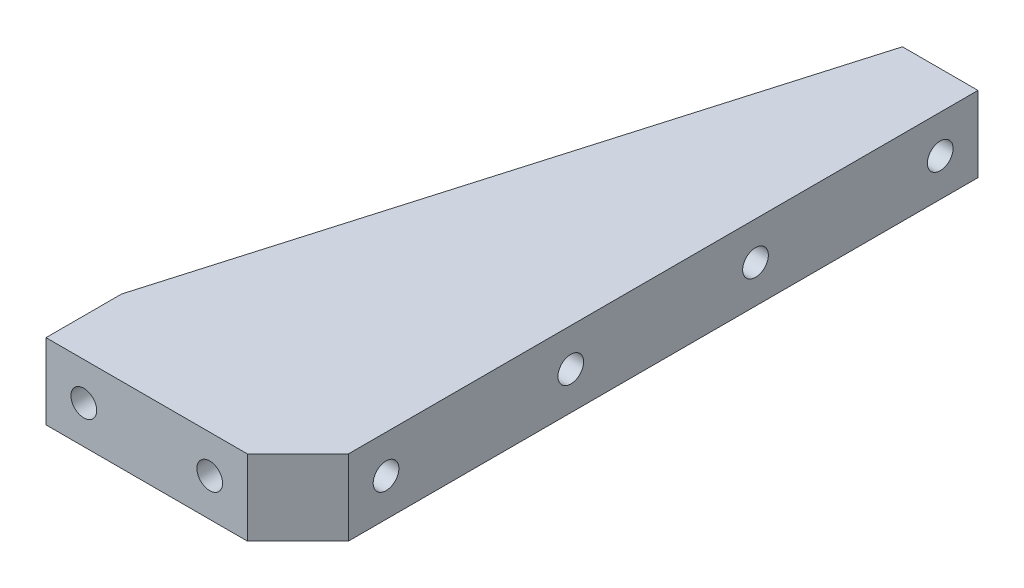
SolidWorks part; units mm, degrees
material "普通碳钢"
ref_plane "前视基准面" through (0, 0, 0) normal (0, 0, 1) x (1, 0, 0)
ref_plane "上视基准面" through (0, 0, 0) normal (0, 1, 0) x (1, 0, 0)
ref_plane "右视基准面" through (0, 0, 0) normal (1, 0, 0) x (0, 0, -1)
sketch "草图1" plane through (0, 0, 0) normal (0, 1, 0) x (1, 0, 0)
  line L0 (0, 0) -> (0, -250)
  line L1 (0, -250) -> (-20, -270)
  line L2 (-20, -270) -> (-100, -270)
  line L3 (-100, -270) -> (-100, -240)
  line L4 (-100, -240) -> (-30, 0)
  line L5 (-30, 0) -> (0, 0)
  dimension "D1" = 270
  dimension "D2" = 100
  dimension "D3" = 30
  dimension "D4" = 30
  dimension "D5" = 45
  dimension "D6" = 20
extrude "凸台-拉伸1" add sketch "草图1" along normal blind 30
hole_wizard "M12 螺纹孔1" positions "草图2" profile "草图3" tap size "M12" standard "GB"
sketch "草图2" plane through (0, 0, 0) normal (1, 0, 0) x (0, 0, -1)
  line L0 (0, 30) -> (0, 0) construction
  line L1 (-250, 30) -> (-250, 0) construction
  line L2 (-15, 15) -> (-88.3333, 15) construction
  line L3 (-88.3333, 15) -> (-161.6667, 15) construction
  line L4 (-161.6667, 15) -> (-235, 15) construction
  point P0 (-235, 15)
  point P2 (-15, 15)
  point P9 (0, 15)
  point P12 (-88.3333, 15)
  point P14 (-161.6667, 15)
  dimension "D1" = 15
  dimension "D2" = 15
sketch "草图3" plane through (0, 15, 235) normal (0, 1, 0) x (0, 0, -1)
  line L0 (0, 0) -> (0, 32.3144)
  line L1 (0, 32.3144) -> (5.1, 29.25)
  line L2 (5.1, 29.25) -> (5.1, 0)
  line L5 (5.1, 0) -> (0, 0)
  line L10 (0, 32.3144) -> (-5.1, 29.25) construction
  line L11 (0, -6.35) -> (0, 107.95) construction
  dimension "螺纹孔钻头直径" = 10.2
  dimension "螺纹孔钻头深度" = 29.25
  dimension "导头角度" = 118
cosmetic thread "孔螺蚊线1"
cosmetic thread "孔螺蚊线2"
cosmetic thread "孔螺蚊线5"
cosmetic thread "孔螺蚊线6"
hole_wizard "M12 螺纹孔2" positions "草图4" profile "草图5" tap size "M12" standard "GB"
sketch "草图4" plane through (0, 0, 270) normal (0, 0, 1) x (1, 0, 0)
  line L0 (-100, 30) -> (-100, 0) construction
  line L1 (-20, 30) -> (-20, 0) construction
  point P0 (-35, 15)
  point P2 (-85, 15)
  point P9 (-100, 15)
  dimension "D1" = 15
  dimension "D2" = 15
sketch "草图5" plane through (-35, 15, 270) normal (1, 0, 0) x (0, -1, 0)
  line L0 (0, 0) -> (0, 32.3144)
  line L1 (0, 32.3144) -> (5.1, 29.25)
  line L2 (5.1, 29.25) -> (5.1, 0)
  line L5 (5.1, 0) -> (0, 0)
  line L10 (0, 32.3144) -> (-5.1, 29.25) construction
  line L11 (0, -6.35) -> (0, 107.95) construction
  dimension "螺纹孔钻头直径" = 10.2
  dimension "螺纹孔钻头深度" = 29.25
  dimension "导头角度" = 118
cosmetic thread "孔螺蚊线3" parameters "D1"=24, "D2"=12
cosmetic thread "孔螺蚊线4" parameters "D1"=24, "D2"=12
